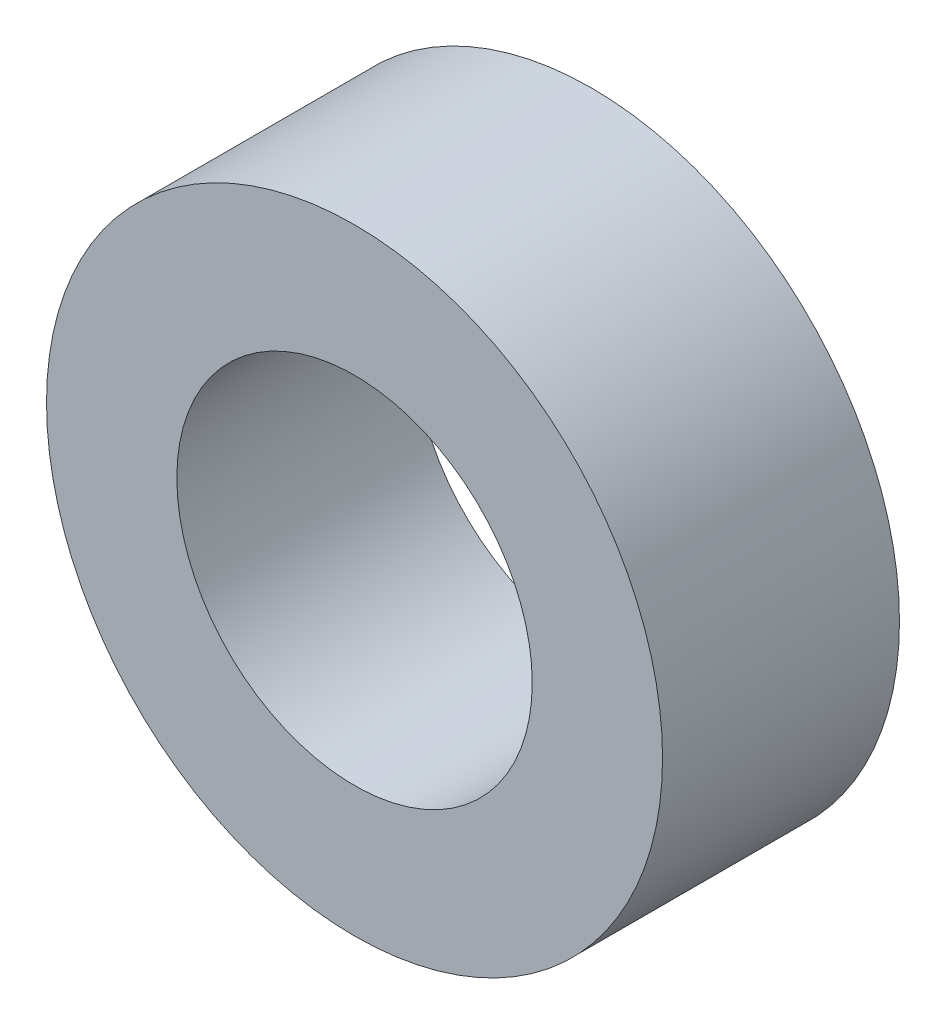
SolidWorks part; units mm, degrees
ref_plane "前视基准面" through (0, 0, 0) normal (0, 0, 1) x (1, 0, 0)
ref_plane "上视基准面" through (0, 0, 0) normal (0, 1, 0) x (1, 0, 0)
ref_plane "右视基准面" through (0, 0, 0) normal (1, 0, 0) x (0, 0, -1)
sketch "草图1" plane through (0, 0, 0) normal (0, 0, 1) x (1, 0, 0)
  circle A0 centre (0, 0) radius 13
  circle A1 centre (0, 0) radius 7.5
  dimension "D1" = 15
  dimension "D2" = 26
extrude "凸台-拉伸1" add sketch "草图1" along normal mid plane 10
